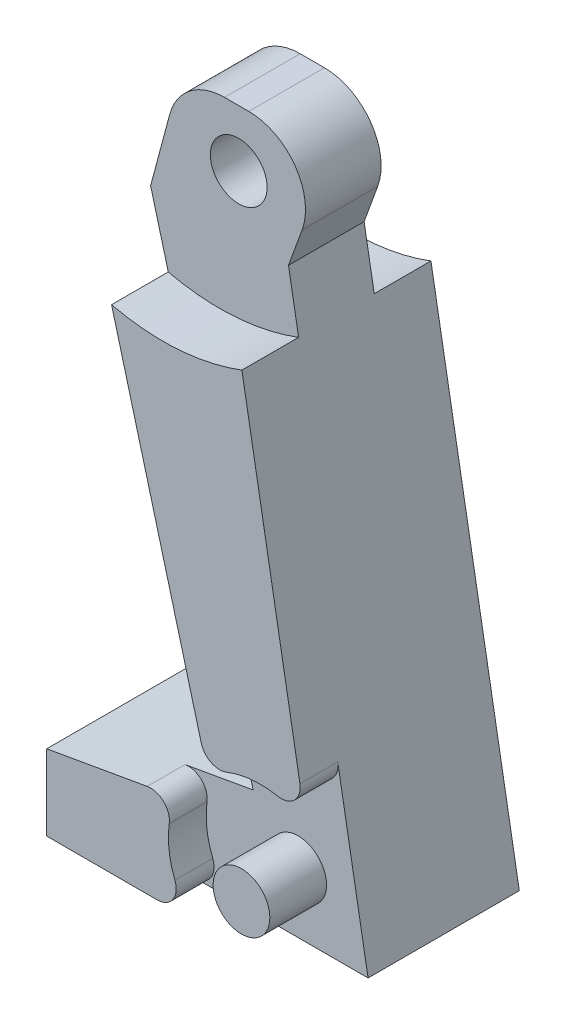
SolidWorks part; units mm, degrees
ref_plane "Front Plane" through (0, 0, 0) normal (0, 0, 1) x (1, 0, 0)
ref_plane "Top Plane" through (0, 0, 0) normal (0, 1, 0) x (1, 0, 0)
ref_plane "Right Plane" through (0, 0, 0) normal (1, 0, 0) x (0, 0, -1)
other "Configuration Table"
sketch "Sketch1" plane through (0, 0, 0) normal (0, 0, 1) x (1, 0, 0)
  line L0 (0, 0) -> (15, 0)
  line L1 (15, 0) -> (9.7906, 29.5442)
  line L2 (9.7906, 29.5442) -> (20.0512, 57.735)
  line L3 (20.0512, 57.735) -> (10.0512, 57.735)
  line L4 (10.0512, 57.735) -> (2.4975, 29.5442)
  line L5 (2.4975, 29.5442) -> (8.9206, 5.5729)
  line L6 (8.9206, 5.5729) -> (0, 4)
  line L7 (0, 4) -> (0, 0)
  dimension "D1" = 15
  dimension "D2" = 80
  dimension "D3" = 30
  dimension "D4" = 150
  dimension "D5" = 30
  dimension "D6" = 10
  dimension "D7" = 105
  dimension "D8" = 150
  dimension "D9" = 85
  dimension "D10" = 4
extrude "Boss-Extrude1" add sketch "Sketch1" along normal blind 10
sketch "Sketch2" plane through (0, 0, 10) normal (0, 0, 1) x (1, 0, 0)
  line L0 (20.0512, 57.735) -> (10.0512, 57.735) construction
  line L1 (8.0512, 87.735) -> (22.0512, 87.735)
  line L2 (8.0512, 87.735) -> (8.0512, 57.735)
  line L3 (8.0512, 57.735) -> (22.0512, 57.735)
  line L4 (22.0512, 87.735) -> (22.0512, 57.735)
  line L5 (15.0512, 57.735) -> (15.0512, 87.735) construction
  line L6 (8.0512, 72.735) -> (22.0512, 72.735) construction
  point P0 (15.0512, 72.735)
  dimension "D1" = 2
  dimension "D2" = 2
  dimension "D3" = 30
extrude "Boss-Extrude2" add sketch "Sketch2" against normal blind 30
ref_plane "Plane1" through (15.0512, 0, 0) normal (-1, 0, 0) x (0, 0, 1)
sketch "Sketch4" plane through (0, 0, 10) normal (0, 0, 1) x (1, 0, 0)
  line L0 (15.0512, 87.735) -> (15.0512, 84.235) construction
  line L1 (22.0512, 87.735) -> (8.0512, 87.735) construction
  line L2 (15.0512, 84.235) -> (30.372, 71.3793)
  line L3 (30.372, 71.3793) -> (30.372, 56.3793)
  line L4 (30.372, 56.3793) -> (27.3079, 56.3793)
  line L5 (27.3079, 56.3793) -> (27.3079, 68.9504)
  line L6 (27.3079, 68.9504) -> (15.0512, 79.235)
  line L7 (15.0512, 79.235) -> (15.0512, 84.235)
  dimension "D1" = 3.5
  dimension "D2" = 5
  dimension "D3" = 50
  dimension "D4" = 20
  dimension "D6" = 16
  dimension "D7" = 15
extrude "Boss-Extrude4" add sketch "Sketch4" along normal blind 5
ref_plane "Plane2" through (0, 0, -5) normal (0, 0, 1) x (1, 0, 0)
mirror "Mirror1" about plane through (0, 0, -5) normal (0, 0, 1) of "Boss-Extrude4", "Boss-Extrude1"
sketch "Sketch5" plane through (0, 87.735, 0) normal (0, 1, 0) x (1, 0, 0)
  line L0 (8.0512, 5) -> (22.0512, 5) construction
  line L1 (8.0512, 20) -> (8.0512, -10) construction
  line L2 (22.0512, 20) -> (22.0512, -10) construction
  line L4 (12.0512, 1.5) -> (18.0512, 1.5)
  line L5 (12.0512, 1.5) -> (12.0512, 8.5)
  line L6 (12.0512, 8.5) -> (18.0512, 8.5)
  line L7 (18.0512, 1.5) -> (18.0512, 8.5)
  line L8 (15.0512, 8.5) -> (15.0512, 1.5) construction
  line L9 (12.0512, 5) -> (18.0512, 5) construction
  point P6 (15.0512, 5)
  dimension "D1" = 6
  dimension "D2" = 7
extrude "Boss-Extrude5" add sketch "Sketch5" along normal blind 6
sketch "Sketch6" plane through (0, 93.735, 0) normal (0, 1, 0) x (1, 0, 0)
  line L0 (15.0512, 8.5) -> (15.0512, 1.5) construction
  line L1 (18.0512, 8.5) -> (12.0512, 8.5) construction
  line L2 (12.0512, 1.5) -> (18.0512, 1.5) construction
  line L4 (7.5512, -2.5) -> (22.5512, -2.5)
  line L5 (7.5512, -2.5) -> (7.5512, 12.5)
  line L6 (7.5512, 12.5) -> (22.5512, 12.5)
  line L7 (22.5512, -2.5) -> (22.5512, 12.5)
  line L8 (15.0512, 12.5) -> (15.0512, -2.5) construction
  line L9 (7.5512, 5) -> (22.5512, 5) construction
  point P6 (15.0512, 5)
  dimension "D1" = 15
  dimension "D2" = 15
extrude "Boss-Extrude6" add sketch "Sketch6" along normal blind 14
sketch "Sketch7" plane through (7.5512, 0, 0) normal (-1, 0, 0) x (0, 0, 1)
  line L0 (-5, 107.735) -> (-5, 93.735) construction
  line L1 (-12.5, 107.735) -> (2.5, 107.735) construction
  line L2 (-8.5, 93.735) -> (-1.5, 93.735) construction
  line L3 (-12.5, 107.735) -> (-12.5, 93.735) construction
  circle A0 centre (-8.96, 103.735) radius 1
  circle A1 centre (-1.04, 103.735) radius 1
  dimension "D1" = 2
  dimension "D2" = 3.54
  dimension "D3" = 4
extrude "Cut-Extrude1" cut sketch "Sketch7" against normal blind 2
fillet "Fillet1" radius 1 10 edges at (18.5512, 81.2982, 10) (18.5512, 76.2982, 10) (18.5512, 81.2982, -20) (18.5512, 76.2982, -20) (15.0512, 81.735, 10) (15.0512, 81.735, -20) (15.0512, 79.235, -22.5) (15.0512, 84.235, -22.5) (15.0512, 79.235, 12.5) (15.0512, 84.235, 12.5)
sketch "Sketch8" plane through (0, 0, -20) normal (0, 0, -1) x (-1, 0, 0)
  line L0 (-9.7906, 29.5442) -> (-20.0512, 57.735) construction
  line L1 (-15, 0) -> (6.2977, 0)
  line L2 (-15, 0) -> (-15, 29.5442)
  line L3 (-15, 29.5442) -> (6.2977, 29.5442)
  line L4 (6.2977, 0) -> (6.2977, 29.5442)
  circle A0 centre (-7.1578, 32.5442) radius 1.5
  dimension "D1" = 3
  dimension "D2" = 3
  dimension "D3" = 3.5
extrude "Cut-Extrude2" cut sketch "Sketch8" against normal blind 10
sketch "Sketch9" plane through (8.0512, 0, 0) normal (-1, 0, 0) x (0, 0, 1)
  line L0 (-15, 29.5442) -> (-15, 57.735) construction
  line L1 (-20, 29.5442) -> (-10, 29.5442) construction
  line L2 (-20, 57.735) -> (-10, 57.735) construction
  line L3 (-10, 57.735) -> (-10, 29.5442) construction
  line L4 (-17, 36.5442) -> (-13, 36.5442)
  line L5 (-17, 36.5442) -> (-17, 24.5442)
  line L6 (-17, 24.5442) -> (-13, 24.5442)
  line L7 (-13, 36.5442) -> (-13, 24.5442)
  line L8 (-15, 24.5442) -> (-15, 36.5442) construction
  line L9 (-17, 30.5442) -> (-13, 30.5442) construction
  point P6 (-15, 30.5442)
  dimension "D1" = 3
  dimension "D2" = 12
  dimension "D3" = 5
extrude "Cut-Extrude3" cut sketch "Sketch9" against normal mid plane 15
sketch "Sketch11" plane through (0, 0, -20) normal (0, 0, -1) x (-1, 0, 0)
  line L0 (-10.0512, 57.735) -> (-2.4975, 29.5442) construction
  line L1 (-4.1052, 35.5442) -> (-50.7872, 35.5442)
  line L2 (-4.1052, 35.5442) -> (-4.1052, 113.6456)
  line L3 (-4.1052, 113.6456) -> (-50.7872, 113.6456)
  line L4 (-50.7872, 35.5442) -> (-50.7872, 113.6456)
  line L5 (-2.4975, 29.5442) -> (-9.7906, 29.5442) construction
  circle A0 centre (-7.1578, 32.5442) radius 1.5 construction
  circle A1 centre (-7.1578, 32.5442) radius 1.5
  dimension "D1" = 6
extrude "Cut-Extrude6" cut sketch "Sketch11" against normal mid plane 100
sketch "Sketch12" plane through (0, 0, -20) normal (0, 0, -1) x (-1, 0, 0)
  line L1 (-21.6998, 42.3416) -> (3.494, 42.3416)
  line L2 (-21.6998, 42.3416) -> (-21.6998, 25.3811)
  line L3 (-21.6998, 25.3811) -> (3.494, 25.3811)
  line L4 (3.494, 42.3416) -> (3.494, 25.3811)
extrude "Cut-Extrude7" cut sketch "Sketch12" against normal blind 20
fillet "Fillet2" radius 3 2 edges at (11.9744, 35.5442, 5) (4.1052, 35.5442, 5)
sketch "Sketch13" plane through (0, 0, 0) normal (1, 0, 0) x (0, 0, -1)
  line L0 (-10, 29.5442) -> (0, 29.5442) construction
  line L1 (-10, 35.5442) -> (-7, 35.5442)
  line L2 (-10, 35.5442) -> (-10, 29.5442)
  line L3 (-10, 29.5442) -> (-7, 29.5442)
  line L4 (-7, 35.5442) -> (-7, 29.5442)
  line L6 (0, 35.5442) -> (-3, 35.5442)
  line L7 (0, 35.5442) -> (0, 29.5442)
  line L8 (0, 29.5442) -> (-3, 29.5442)
  line L9 (-3, 35.5442) -> (-3, 29.5442)
  dimension "D1" = 3
extrude "Cut-Extrude8" cut sketch "Sketch13" along normal blind 20
fillet "Fillet3" [suppressed] radius 3
fillet "Fillet4" [suppressed] radius 3
sketch "Sketch14" plane through (0, 0, 0) normal (0, 0, -1) x (-1, 0, 0)
  line L0 (-6.144, 29.5442) -> (-6.144, 37.5442)
  line L1 (-9.7906, 29.5442) -> (-2.4975, 29.5442) construction
  circle A0 centre (-6.144, 37.5442) radius 11.8
  line M2 (-2.4975, 29.5442) -> (-9.7906, 29.5442)
  dimension "D1" = 8
extrude "Cut-Extrude9" cut sketch "Sketch14" against normal blind 3 contours A0 M2
ref_plane "Plane3" through (0, 0, 5) normal (0, 0, -1) x (-1, 0, 0)
mirror "Mirror2" about plane through (0, 0, 5) normal (0, 0, -1) of "Cut-Extrude9"
sketch "Sketch15" plane through (0, 0, 10) normal (0, 0, 1) x (1, 0, 0)
  circle A0 centre (11.3032, 3.1632) radius 1.5
  dimension "D1" = 3
extrude "Boss-Extrude7" add sketch "Sketch15" along normal blind 1
sketch "Sketch16" plane through (0, 0, 10) normal (0, 0, 1) x (1, 0, 0)
  circle A0 centre (11.3032, 3.1632) radius 4.8653
  circle A1 centre (11.3032, 3.1632) radius 1.5 construction
  circle A2 centre (11.3032, 3.1632) radius 1.5
extrude "Cut-Extrude10" cut sketch "Sketch16" against normal blind 2
fillet "Fillet5" radius 1 4 edges at (7.6065, 0, 9) (6.8918, 5.2152, 9) (8.5006, 7.1402, 9) (13.6952, 7.3999, 9)
sketch "Sketch17" [suppressed] plane through (30.372, 0, 0) normal (1, 0, 0) x (0, 0, -1)
  line L0 (-15, 56.3793) -> (-10, 56.3793) construction
  line L1 (-15, 56.3793) -> (-15, 71.3793) construction
  line L2 (25, 56.3793) -> (25, 71.3793) construction
  circle A0 centre (-12.5, 58.8793) radius 1.5
  circle A1 centre (22.5, 58.8793) radius 1.5
  dimension "D1" = 3
  dimension "D2" = 2.5
  dimension "D3" = 2.5
  dimension "D4" = 3
  dimension "D5" = 2.5
extrude "Cut-Extrude11" [suppressed] cut sketch "Sketch17" against normal blind 6
